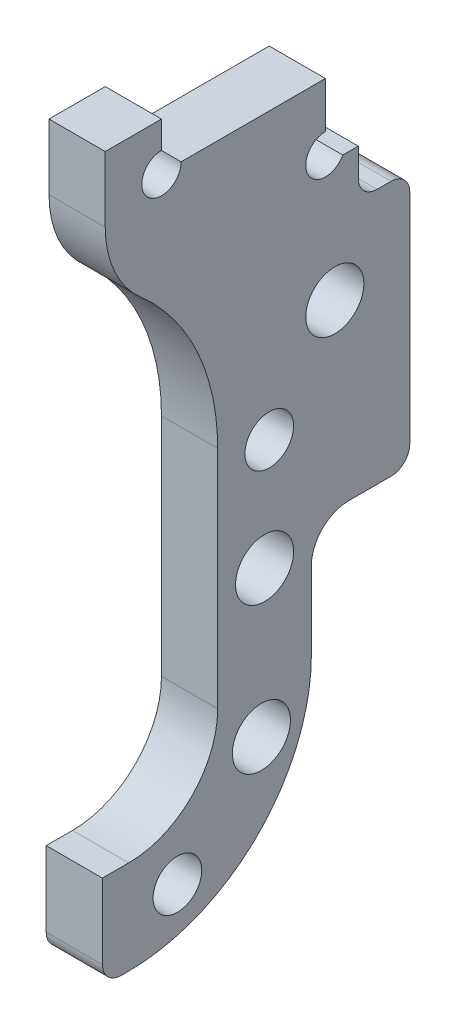
from build123d import *

# Parameters (mm, degrees)
SKETCH_1_R      = 1.55
SKETCH_1_R_2    = 1.3
EXTRUDE_1_DEPTH = 3
SKETCH_2_W      = 0.25
SKETCH_2_H      = 13.633784975
EXTRUDE_2_DEPTH = 3
FILLET_R2_1_R   = 2
FILLET_R1_1_R   = 1


with BuildPart() as part:
    # 草图1 → 凸台-拉伸1 (new body)
    with BuildSketch(Plane(origin=(0, 0, 0), x_dir=(0, 0, -1), z_dir=(1, 0, 0))):
        with BuildLine():
            Line((-14.25, 6.116215025), (-9.25, 6.116215025))
            Line((-9.25, 6.116215025), (-9.25, 19.75))
            Line((-9.25, 19.75), (-19.25, 19.75))
            Line((-19.25, 19.75), (-19.25, 0))
            ThreePointArc((-19.25, 0), (-20.641242789, -3.358757211), (-24, -4.75))
            Line((-24, -4.75), (-25.4, -4.75))
            Line((-25.4, -4.75), (-25.4, -9.75))
            Line((-25.4, -9.75), (-24, -9.75))
            ThreePointArc((-24, -9.75), (-17.105708883, -6.894291117), (-14.25, 0))
            Line((-14.25, 0), (-14.25, 6.116215025))
        make_face()
        with Locations((-13, 15.75)):
            Circle(SKETCH_1_R, mode=Mode.SUBTRACT)
        with Locations((-16.75, 5.25)):
            Circle(SKETCH_1_R, mode=Mode.SUBTRACT)
        with Locations((-16.5, 11.05)):
            Circle(SKETCH_1_R_2, mode=Mode.SUBTRACT)
        with Locations((-21.4, -7.034912935)):
            Circle(SKETCH_1_R_2, mode=Mode.SUBTRACT)
        with Locations((-16.917350474, -2.466997302)):
            Circle(SKETCH_1_R, mode=Mode.SUBTRACT)
    extrude(amount=EXTRUDE_1_DEPTH)

    # 草图2 → 凸台-拉伸2 (add, through all)
    with BuildSketch(Plane(origin=(3, 0, 0), x_dir=(0, 0, -1), z_dir=(1, 0, 0))):
        with BuildLine():
            Line((-19.25, 19.75), (-11.75, 19.75))
            Line((-11.75, 19.75), (-11.75, 22.25))
            Line((-11.75, 22.25), (-12.576690734, 22.25))
            ThreePointArc((-12.576690734, 22.25), (-14.402080928, 22.212645368), (-13.5, 23.8))
            Line((-13.5, 23.8), (-13.5, 26.25))
            Line((-13.5, 26.25), (-21.2, 26.25))
            ThreePointArc((-21.2, 26.25), (-22.99246212, 25.50753788), (-22.25, 27.3))
            Line((-22.25, 27.3), (-22.25, 28.75))
            Line((-22.25, 28.75), (-25.25, 28.75))
            Line((-25.25, 28.75), (-25.25, 25.25))
            ThreePointArc((-25.25, 25.25), (-24.753426104, 22.95535741), (-23.352564103, 21.071330896))
            ThreePointArc((-23.352564103, 21.071330896), (-20.323673289, 16.997760056), (-19.25, 12.036370673))
            Line((-19.25, 12.036370673), (-19.25, 19.75))
        make_face()
        with Locations((-9.125, 12.933107513)):
            Rectangle(SKETCH_2_W, SKETCH_2_H)
    extrude(amount=-EXTRUDE_2_DEPTH)

    # R2 圆角1
    fillet_r2_1_edges = [part.edges().sort_by_distance(p)[0] for p in [
        (1.5, 6.116215025, 14.25),
    ]]
    fillet(fillet_r2_1_edges, radius=FILLET_R2_1_R)

    # R1 圆角1
    fillet_r1_1_edges = [part.edges().sort_by_distance(p)[0] for p in [
        (1.5, -9.75, 25.4),
        (1.5, 19.75, 11.75),
        (1.5, 19.75, 9),
        (1.5, 6.116215025, 9),
    ]]
    fillet(fillet_r1_1_edges, radius=FILLET_R1_1_R)


solid = part.part
